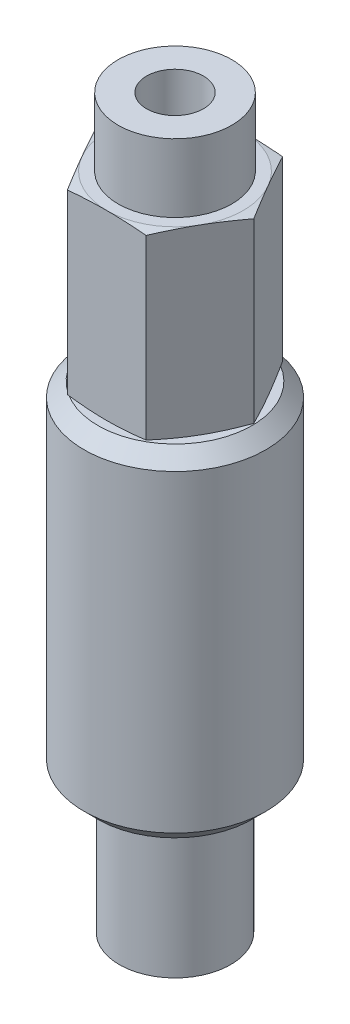
from build123d import *

# Parameters (mm, degrees)
SKETCH_2_R          = 6
CUT_EXTRUDE_1_DEPTH = 8
SKETCH_3_W          = 2.5
SKETCH_3_H          = 3
SKETCH_4_W          = 1.25
SKETCH_4_H          = 32


with BuildPart() as part:
    # 草图1 → 旋转1 (revolve)
    with BuildSketch(Plane.XY, mode=Mode.PRIVATE) as revolve_1_sk:
        Polygon((0, 41), (3, 41), (5, 40.647346039), (5, 33.535898385), (3, 33), (3.3865, 33), (4, 32.3865), (4, 18.6135), (3.3865, 18), (2.45, 18), (2.45, 12), (0, 12), align=None)
    revolve(revolve_1_sk.sketch.rotate(Axis((0, 12, 0), (0, 1, 0)), 180), axis=Axis((0, 12, 0), (0, 1, 0)))

    # 草图2 → 切除-拉伸1 (cut)
    with BuildSketch(Plane(origin=(0, 33, 0), x_dir=(1, 0, 0), z_dir=(0, 1, 0))):
        Circle(SKETCH_2_R)
        Polygon((-3.464101615, 0), (-1.732050808, -3), (1.732050808, -3), (3.464101615, 0), (1.732050808, 3), (-1.732050808, 3), align=None, mode=Mode.SUBTRACT)
    extrude(amount=CUT_EXTRUDE_1_DEPTH, mode=Mode.SUBTRACT)

    # 草图3 → 旋转2 (revolve)
    with BuildSketch(Plane.XY, mode=Mode.PRIVATE) as revolve_2_sk:
        with Locations((1.25, 42.5)):
            Rectangle(SKETCH_3_W, SKETCH_3_H)
    revolve(revolve_2_sk.sketch.rotate(Axis((0, 41, 0), (0, 1, 0)), 270), axis=Axis((0, 41, 0), (0, 1, 0)))

    # 草图4 → 切除-旋转1 (revolve, cut)
    with BuildSketch(Plane.XY, mode=Mode.PRIVATE) as cut_revolve_1_sk:
        with Locations((0.625, 28)):
            Rectangle(SKETCH_4_W, SKETCH_4_H)
    revolve(cut_revolve_1_sk.sketch.rotate(Axis((0, 12, 0), (0, 1, 0)), 270), axis=Axis((0, 12, 0), (0, 1, 0)), mode=Mode.SUBTRACT)


solid = part.part
